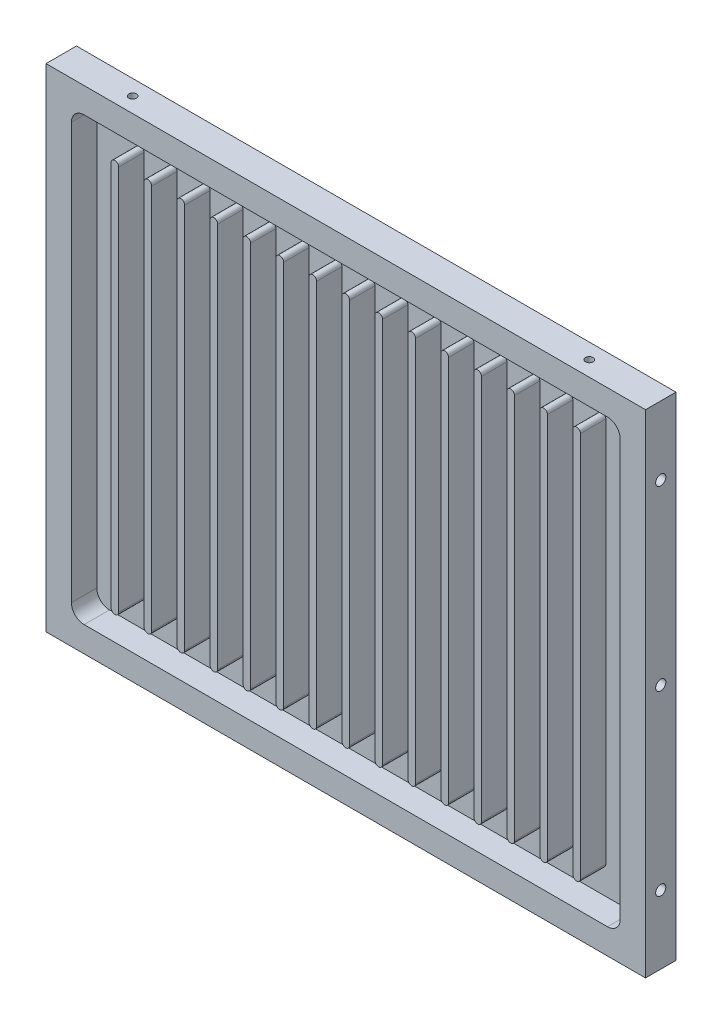
from build123d import *

# Parameters (mm, degrees)
SKETCH1_W           = 236.3
SKETCH1_H           = 194
BOSS_EXTRUDE1_DEPTH = 6
SKETCH2_W           = 216.3
SKETCH2_H           = 174
CUT_EXTRUDE1_DEPTH  = 10
BOSS_EXTRUDE2_DEPTH = 10
LPATTERN1_COUNT     = 8
LPATTERN1_PITCH     = 13
LPATTERN1_COL_COUNT = 8
LPATTERN1_COL_PITCH = 13
SKETCH5_R           = 1.5
CUT_EXTRUDE2_DEPTH  = 4
SKETCH6_R           = 2
CUT_EXTRUDE3_DEPTH  = 4
FILLET1_R           = 5


with BuildPart() as part:
    # Sketch1 → Boss-Extrude1 (new, symmetric)
    with BuildSketch(Plane.XY):
        Rectangle(SKETCH1_W, SKETCH1_H)
    extrude(amount=BOSS_EXTRUDE1_DEPTH, both=True)

    # Sketch2 → Cut-Extrude1 (cut)
    with BuildSketch(Plane.XY.offset(6)):
        Rectangle(SKETCH2_W, SKETCH2_H)
    extrude(amount=-CUT_EXTRUDE1_DEPTH, mode=Mode.SUBTRACT)

    # Sketch3 → Boss-Extrude2 (add)
    with BuildSketch(Plane.XY.offset(-4)):
        with BuildLine():
            Line((-1.5, 76), (-1.5, -76))
            ThreePointArc((-1.5, -76), (0, -77.5), (1.5, -76))
            Line((1.5, -76), (1.5, 76))
            ThreePointArc((1.5, 76), (0, 77.5), (-1.5, 76))
        make_face()
    boss_extrude2 = extrude(amount=BOSS_EXTRUDE2_DEPTH)

    # LPattern1: Boss-Extrude2 ×8
    with Locations(*[(i * LPATTERN1_PITCH, 0, 0) for i in range(1, LPATTERN1_COUNT)]):
        add(boss_extrude2)

    # LPattern1 col: Boss-Extrude2 ×8
    with Locations(*[(-i * LPATTERN1_COL_PITCH, 0, 0) for i in range(1, LPATTERN1_COL_COUNT)]):
        add(boss_extrude2)

    # Sketch5 → Cut-Extrude2 (cut)
    with BuildSketch(Plane(origin=(0, 97, 0), x_dir=(1, 0, 0), z_dir=(0, 1, 0))):
        with Locations(Location((-90, 0, 0), (0, 0, 270))):
            Circle(SKETCH5_R)
        with Locations(Location((90, 0, 0), (0, 0, 90))):
            Circle(SKETCH5_R)
    cut_extrude2 = extrude(amount=-CUT_EXTRUDE2_DEPTH, mode=Mode.SUBTRACT)

    # Mirror1: Cut-Extrude2 across plane
    add(cut_extrude2.mirror(Plane.ZX), mode=Mode.SUBTRACT)

    # Sketch6 → Cut-Extrude3 (cut)
    with BuildSketch(Plane.ZY.offset(118.15)):
        with Locations(Location((0, 70, 0), (0, 0, 270))):
            Circle(SKETCH6_R)
        with Locations(Location((0, 0, 0), (0, 0, 270))):
            Circle(SKETCH6_R)
        with Locations(Location((0, -70, 0), (0, 0, 90))):
            Circle(SKETCH6_R)
    cut_extrude3 = extrude(amount=-CUT_EXTRUDE3_DEPTH, mode=Mode.SUBTRACT)

    # Mirror2: Cut-Extrude3 across plane
    add(cut_extrude3.mirror(Plane(origin=(0, 0, 0), x_dir=(0, 0, 1), z_dir=(1, 0, 0))), mode=Mode.SUBTRACT)

    # Fillet1
    fillet1_edges = [part.edges().sort_by_distance(p)[0] for p in [
        (-108.15, 87, 1),
        (108.15, 87, 1),
        (108.15, -87, 1),
        (-108.15, -87, 1),
    ]]
    fillet(fillet1_edges, radius=FILLET1_R)


solid = part.part
